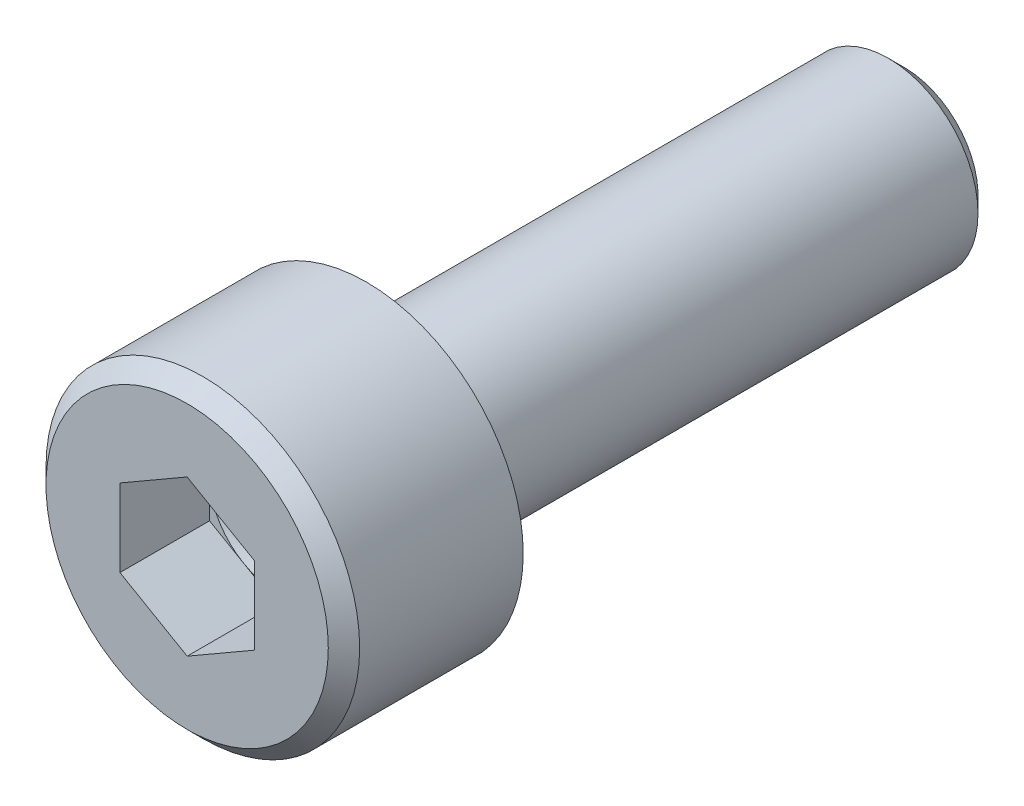
SolidWorks part; units mm, degrees
material "SUS304/0Cr18Ni9"
ref_plane "前视基准面" through (0, 0, 0) normal (0, 0, 1) x (1, 0, 0)
ref_plane "上视基准面" through (0, 0, 0) normal (0, 1, 0) x (1, 0, 0)
ref_plane "右视基准面" through (0, 0, 0) normal (1, 0, 0) x (0, 0, -1)
sketch "草图1" plane through (0, 0, 0) normal (0, 1, 0) x (1, 0, 0)
  line L0 (3.5, 0) -> (0, 0)
  line L1 (0, 0) -> (0, -4)
  line L2 (0, -4) -> (3.5, -4)
  line L3 (3.5, -4) -> (3.5, 0)
  line L4 (0, 0) -> (0, -4) construction
revolve "旋转1" add sketch "草图1" angle 360 about L4
sketch "草图2" plane through (0, 0, 0) normal (0, 0, -1) x (-1, 0, 0)
  circle A0 centre (0, 0) radius 2
extrude "凸台-拉伸1" add sketch "草图2" along normal blind 12
sketch "草图3" plane through (0, 0, 4) normal (0, 0, 1) x (1, 0, 0)
  line L0 (1.5, -0.866) -> (1.5, 0.866)
  line L1 (1.5, 0.866) -> (0, 1.7321)
  line L2 (0, 1.7321) -> (-1.5, 0.866)
  line L3 (-1.5, 0.866) -> (-1.5, -0.866)
  line L4 (-1.5, -0.866) -> (0, -1.7321)
  line L5 (0, -1.7321) -> (1.5, -0.866)
extrude "切除-拉伸1" cut sketch "草图3" against normal blind 2
ref_plane "基准面1" through (0, 0, 0) normal (0, -1, 0) x (1, 0, 0)
sketch "草图4" plane through (0, 0, 0) normal (0, -1, 0) x (1, 0, 0)
  line L0 (1.5, 2) -> (0, 2)
  line L1 (0, 2) -> (0, 1.134)
  line L2 (0, 1.134) -> (1.5, 2)
  line L3 (0, 2) -> (0, 1.134) construction
revolve "切除-旋转1" cut sketch "草图4" angle 360 about L3
chamfer "倒角1" distance 0.35 angle 45 2 edges at (-2, 0, -12) (3.5, 0, 4)
